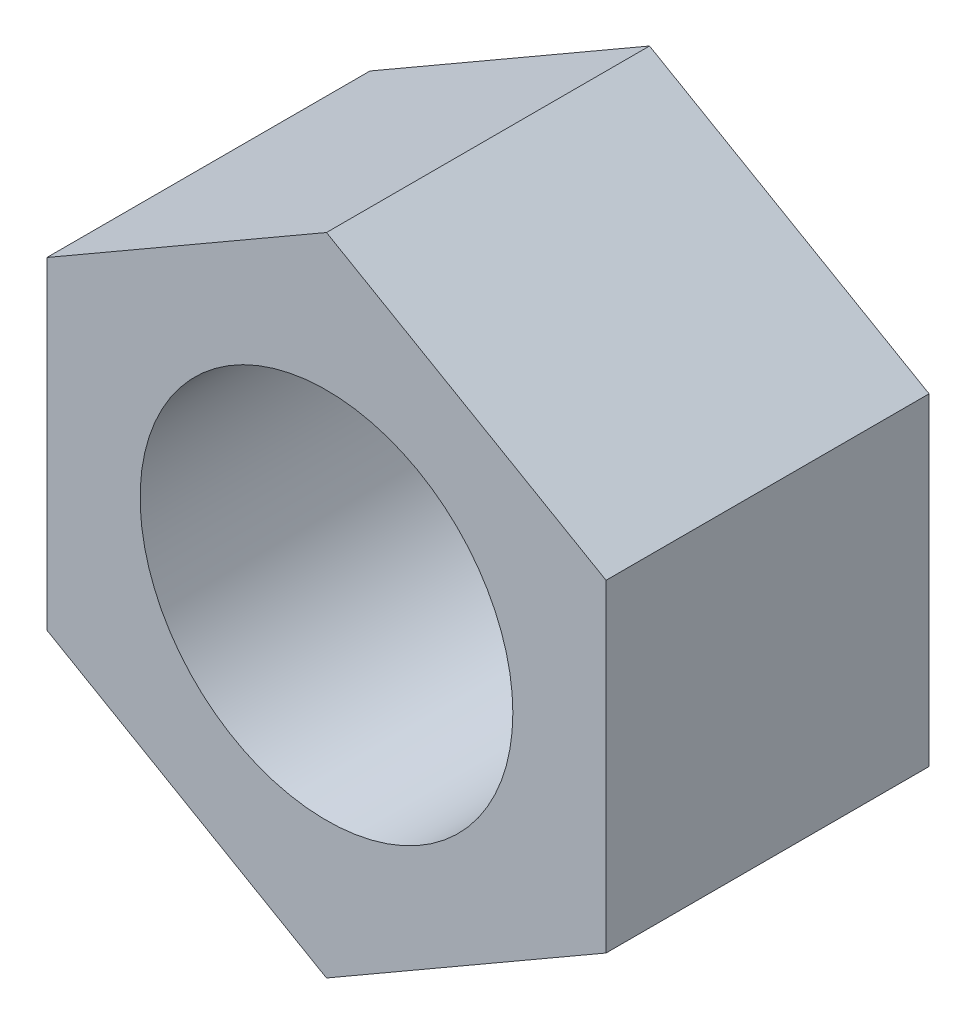
SolidWorks part; units mm, degrees
ref_plane "Front Plane" through (0, 0, 0) normal (0, 0, 1) x (1, 0, 0)
ref_plane "Top Plane" through (0, 0, 0) normal (0, 1, 0) x (1, 0, 0)
ref_plane "Right Plane" through (0, 0, 0) normal (1, 0, 0) x (0, 0, -1)
sketch "Sketch1" plane through (0, 0, 0) normal (0, 0, 1) x (1, 0, 0)
  line L1 (0, -10.3923) -> (9, -5.1962)
  line L2 (9, -5.1962) -> (9, 5.1962)
  line L3 (9, 5.1962) -> (0, 10.3923)
  line L4 (0, 10.3923) -> (-9, 5.1962)
  line L5 (-9, 5.1962) -> (-9, -5.1962)
  line L6 (-9, -5.1962) -> (0, -10.3923)
  circle A0 centre (0, 0) radius 9 construction
  circle A1 centre (0, 0) radius 6
  dimension "D1" = 18
  dimension "D2" = 12
extrude "Boss-Extrude1" add sketch "Sketch1" along normal blind 10.4
cosmetic thread "Cosmetic Thread1"
